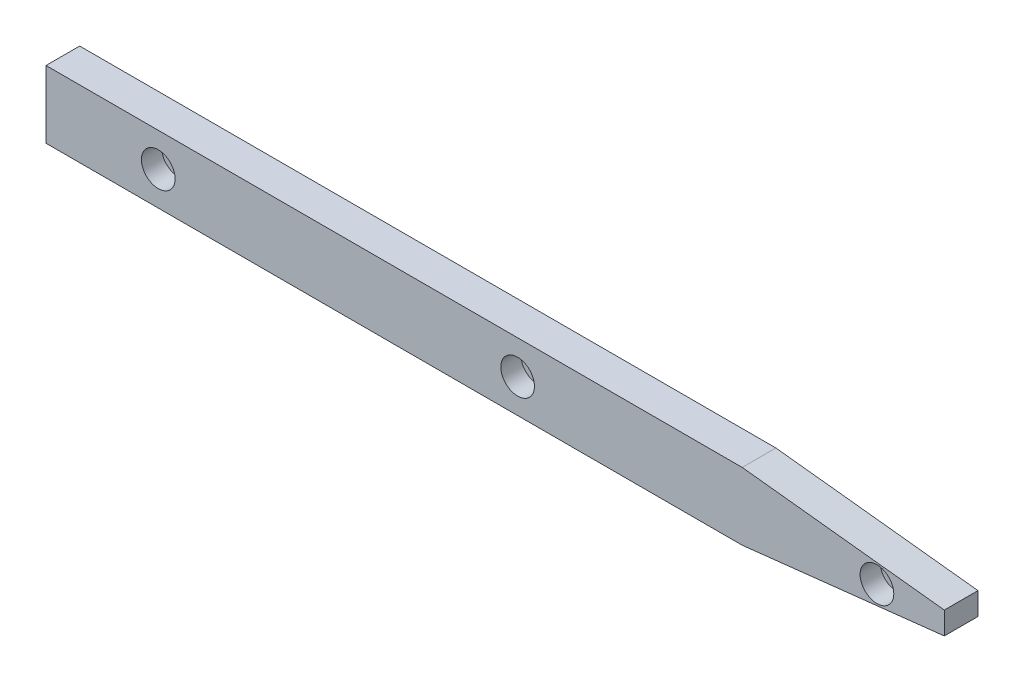
SolidWorks part; units mm, degrees
material "6061 合金"
ref_plane "前视基准面" through (0, 0, 0) normal (0, 0, 1) x (1, 0, 0)
ref_plane "上视基准面" through (0, 0, 0) normal (0, 1, 0) x (1, 0, 0)
ref_plane "右视基准面" through (0, 0, 0) normal (1, 0, 0) x (0, 0, -1)
sketch "草图1" plane through (0, 0, 0) normal (0, 0, 1) x (1, 0, 0)
  line L0 (200, 5) -> (110, 15)
  line L1 (110, -15) -> (-200, -15)
  line L2 (200, -5) -> (200, 5)
  line L3 (110, 15) -> (-200, 15)
  line L4 (-200, -15) -> (-200, 15)
  line L5 (200, -15) -> (-200, 15) construction
  line L6 (200, 15) -> (-200, -15) construction
  line L7 (110, -15) -> (200, -5)
  point P0 (0, 0)
  dimension "D1" = 30
  dimension "D2" = 400
  dimension "D3" = 10
  dimension "D4" = 90
  dimension "D5" = 10
  dimension "D6" = 90
extrude "凸台-拉伸1" add sketch "草图1" along normal mid plane 15
hole_wizard "M8 螺纹孔1" positions "3D草图1" profile "草图2" tap size "M8" standard "GB"
sketch3d "3D草图1"
  line L0 (-200, 15, 7.5) -> (-200, 15, -7.5) construction
  line L2 (-200, 15, 7.5) -> (-200, -15, 7.5) construction
  point P0 (-200, 0, 0)
  dimension "D1" = 15
  dimension "D4" = 7.5
sketch "草图2" plane through (-200, 0, 0) normal (0, 1, 0) x (0, 0, 1)
  line L0 (0, 0) -> (0, 21.7929)
  line L1 (0, 21.7929) -> (3.4, 19.75)
  line L2 (3.4, 19.75) -> (3.4, 0)
  line L5 (3.4, 0) -> (0, 0)
  line L10 (0, 21.7929) -> (-3.4, 19.75) construction
  line L11 (0, -6.35) -> (0, 107.95) construction
  dimension "螺纹孔钻头直径" = 6.8
  dimension "螺纹孔钻头深度" = 19.75
  dimension "导头角度" = 118
cosmetic thread "孔螺蚊线2" parameters "D1"=16, "D2"=8
hole_wizard "打孔尺寸(%根据)内六角圆柱头螺钉的类型1" positions "3D草图2" profile "草图3" counterbore size "M8" standard "GB"
sketch3d "3D草图2"
  line L0 (-200, 15, 7.5) -> (-200, -15, 7.5) construction
  line L1 (-200, -15, 7.5) -> (110, -15, 7.5) construction
  point P0 (-150, 0, 7.5)
  point P2 (0, 0, 0)
  point P5 (170, 0, 7.5)
  point P7 (10, 0, 7.5)
  dimension "D1" = 160
  dimension "D2" = 160
  dimension "D3" = 50
  dimension "D4" = 15
  dimension "D5" = 15
  dimension "D6" = 15
sketch "草图3" plane through (-150, 0, 7.5) normal (1, 0, 0) x (0, -1, 0)
  line L0 (0, 0) -> (0, 15)
  line L1 (0, 15) -> (4.5, 15)
  line L3 (4.5, 15) -> (4.5, 9)
  line L4 (4.5, 9) -> (7.5, 9)
  line L5 (7.5, 9) -> (7.5, 0)
  line L7 (7.5, 0) -> (0, 0)
  line L11 (0, -6.35) -> (0, 107.95) construction
  dimension "通孔孔直径" = 9
  dimension "通孔孔深度" = 15
  dimension "柱形沉头孔直径" = 15
  dimension "柱形沉头孔深度" = 9
